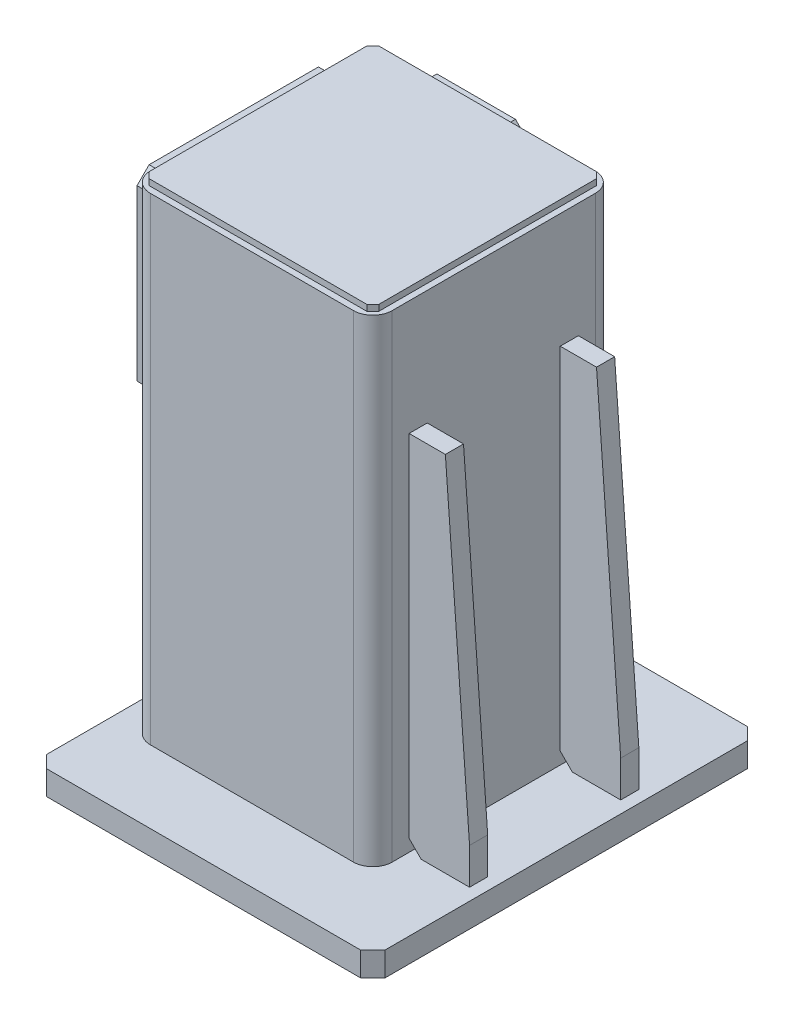
from build123d import *

# Parameters (mm, degrees)
BOSS_EXTRUDE1_DEPTH = 20
BOSS_EXTRUDE2_DEPTH = 395
BOSS_EXTRUDE3_START = -30
BOSS_EXTRUDE3_DEPTH = 15
BOSS_EXTRUDE4_DEPTH = 5
BOSS_EXTRUDE5_DEPTH = 15
CHAMFER1_SIZE       = 10
BOSS_EXTRUDE8_DEPTH = 20
FILLET1_R           = 5
CHAMFER2_SIZE       = 10


with BuildPart() as part:
    # Sketch1 → Boss-Extrude1 (new body)
    with BuildSketch(Plane(origin=(0, 0, 0), x_dir=(1, 0, 0), z_dir=(0, 1, 0))):
        Polygon((280, 0), (280, -320), (0, -320), (0, -50), (135, -50), (135, 0), align=None)
    extrude(amount=BOSS_EXTRUDE1_DEPTH)

    # Sketch2 → Boss-Extrude2 (add)
    with BuildSketch(Plane(origin=(0, 20, 0), x_dir=(1, 0, 0), z_dir=(0, 1, 0))):
        with BuildLine():
            Line((36, -60), (204, -60))
            ThreePointArc((204, -60), (215.313708499, -64.686291501), (220, -76))
            Line((220, -76), (220, -244))
            ThreePointArc((220, -244), (215.313708499, -255.313708499), (204, -260))
            Line((204, -260), (36, -260))
            ThreePointArc((36, -260), (24.686291501, -255.313708499), (20, -244))
            Line((20, -244), (20, -76))
            ThreePointArc((20, -76), (24.686291501, -64.686291501), (36, -60))
        make_face()
        with BuildLine():
            Line((36, -68), (204, -68))
            ThreePointArc((204, -68), (209.656854249, -70.343145751), (212, -76))
            Line((212, -76), (212, -244))
            ThreePointArc((212, -244), (209.656854249, -249.656854249), (204, -252))
            Line((204, -252), (36, -252))
            ThreePointArc((36, -252), (30.343145751, -249.656854249), (28, -244))
            Line((28, -244), (28, -76))
            ThreePointArc((28, -76), (30.343145751, -70.343145751), (36, -68))
        make_face(mode=Mode.SUBTRACT)
    extrude(amount=BOSS_EXTRUDE2_DEPTH)

    # Sketch3 → Boss-Extrude3 (add)
    with BuildSketch(Plane.XY.offset(260).offset(BOSS_EXTRUDE3_START)):
        Polygon((230, 20), (270, 20), (270, 50), (250, 320), (220, 320), (220, 30), align=None)
    boss_extrude3 = extrude(amount=-BOSS_EXTRUDE3_DEPTH)

    # Mirror1: Boss-Extrude3 across plane
    add(boss_extrude3.mirror(Plane(origin=(0, 0, 160), x_dir=(1, 0, 0), z_dir=(0, 0, -1))))

    # Sketch4 → Boss-Extrude4 (add)
    with BuildSketch(Plane(origin=(0, 415, 0), x_dir=(1, 0, 0), z_dir=(0, 1, 0))):
        Polygon((30, -65), (210, -65), (215, -70), (215, -250), (210, -255), (30, -255), (25, -250), (25, -70), align=None)
    extrude(amount=BOSS_EXTRUDE4_DEPTH)

    # Sketch5 → Boss-Extrude5 (add)
    with BuildSketch(Plane.ZY.offset(-20)):
        Polygon((90, 405), (230, 405), (240, 395), (240, 255), (230, 245), (90, 245), (80, 255), (80, 395), align=None)
    extrude(amount=BOSS_EXTRUDE5_DEPTH)

    # Chamfer1
    chamfer1_edges = [part.edges().sort_by_distance(p)[0] for p in [
        (280, 10, 0),
        (280, 10, 320),
        (0, 10, 320),
        (0, 10, 50),
    ]]
    chamfer(chamfer1_edges, length=CHAMFER1_SIZE)

    # Sketch8 → Boss-Extrude8 (add)
    with BuildSketch(Plane(origin=(0, 0, 60), x_dir=(-1, 0, 0), z_dir=(0, 0, -1))):
        Polygon((-118, 399), (-53, 399), (-43, 389), (-43, 59), (-53, 49), (-118, 49), (-128, 59), (-128, 389), align=None)
    extrude(amount=BOSS_EXTRUDE8_DEPTH)

    # Fillet1
    fillet1_edges = [part.edges().sort_by_distance(p)[0] for p in [
        (135, 10, 50),
    ]]
    fillet(fillet1_edges, radius=FILLET1_R)

    # Chamfer2
    chamfer2_edges = [part.edges().sort_by_distance(p)[0] for p in [
        (135, 10, 0),
    ]]
    chamfer(chamfer2_edges, length=CHAMFER2_SIZE)


solid = part.part
